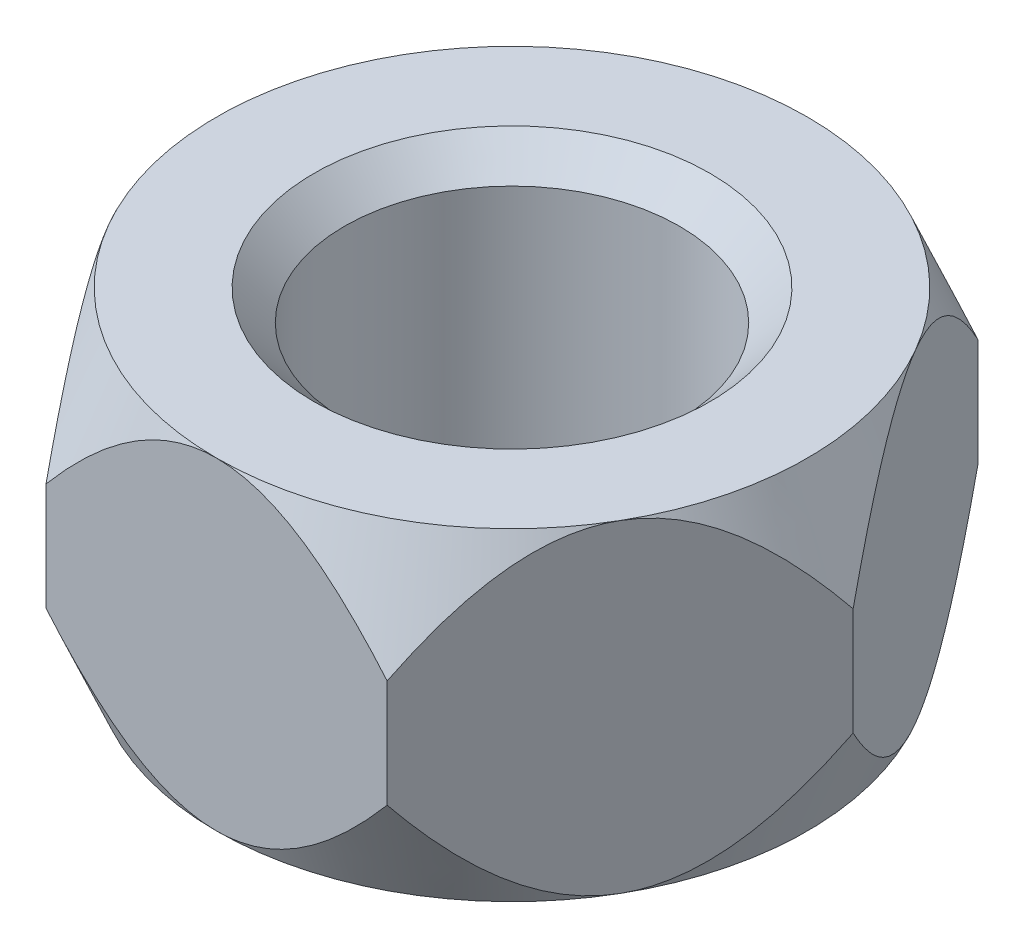
SolidWorks part; units mm, degrees
ref_plane "Front Plane" through (0, 0, 0) normal (0, 0, 1) x (1, 0, 0)
ref_plane "Top Plane" through (0, 0, 0) normal (0, 1, 0) x (1, 0, 0)
ref_plane "Right Plane" through (0, 0, 0) normal (1, 0, 0) x (0, 0, -1)
sketch "Sketch1" plane through (0, 0, 0) normal (0, 1, 0) x (1, 0, 0)
  line L1 (4.3301, 7.5) -> (-4.3301, 7.5)
  line L2 (-4.3301, 7.5) -> (-8.6603, 0)
  line L3 (-8.6603, 0) -> (-4.3301, -7.5)
  line L4 (-4.3301, -7.5) -> (4.3301, -7.5)
  line L5 (4.3301, -7.5) -> (8.6603, 0)
  line L6 (8.6603, 0) -> (4.3301, 7.5)
  circle A0 centre (0, 0) radius 7.5 construction
  dimension "D1" = 15
extrude "Boss-Extrude1" add sketch "Sketch1" along normal blind 8.2
sketch "Sketch2" plane through (0, 8.2, 0) normal (0, 1, 0) x (1, 0, 0)
  line L0 (8.6603, 0) -> (4.3301, 7.5) construction
  circle A0 centre (0, 0) radius 7.5
extrude "Cut-Extrude1" cut sketch "Sketch2" against normal blind 8.2 draft 23 flip side to cut
sketch "Sketch3" plane through (0, 0, 0) normal (0, -1, 0) x (1, 0, 0)
  line L0 (4.3301, 7.5) -> (8.6603, 0) construction
  circle A0 centre (0, 0) radius 7.5
extrude "Cut-Extrude2" cut sketch "Sketch3" against normal blind 8.2 draft 23 flip side to cut
hole_wizard "M10 Tapped Hole1" positions "Sketch4" profile "Sketch5" tap size "M10" standard "GB" end condition through all
sketch "Sketch4" plane through (0, 8.2, 0) normal (0, 1, 0) x (1, 0, 0)
  point P0 (0, 0)
sketch "Sketch5" plane through (0, 8.2, 0) normal (1, 0, 0) x (0, 0, 1)
  line L0 (0, 0) -> (0, 8.2)
  line L1 (0, 8.2) -> (4.25, 8.2)
  line L2 (4.25, 8.2) -> (4.25, 0.775)
  line L3 (4.25, 0.775) -> (5.025, 0)
  line L5 (5.025, 0) -> (0, 0)
  line L6 (-4.25, 0.775) -> (-5.025, 0) construction
  line L11 (0, -6.35) -> (0, 107.95) construction
  dimension "通孔螺纹孔钻头直径" = 8.5
  dimension "通孔螺纹孔钻头深度" = 8.2
  dimension "近端锥形沉头孔直径" = 10.05
  dimension "近端锥形沉头孔角度" = 90
cosmetic thread "Cosmetic Thread1" parameters "D2"=10
